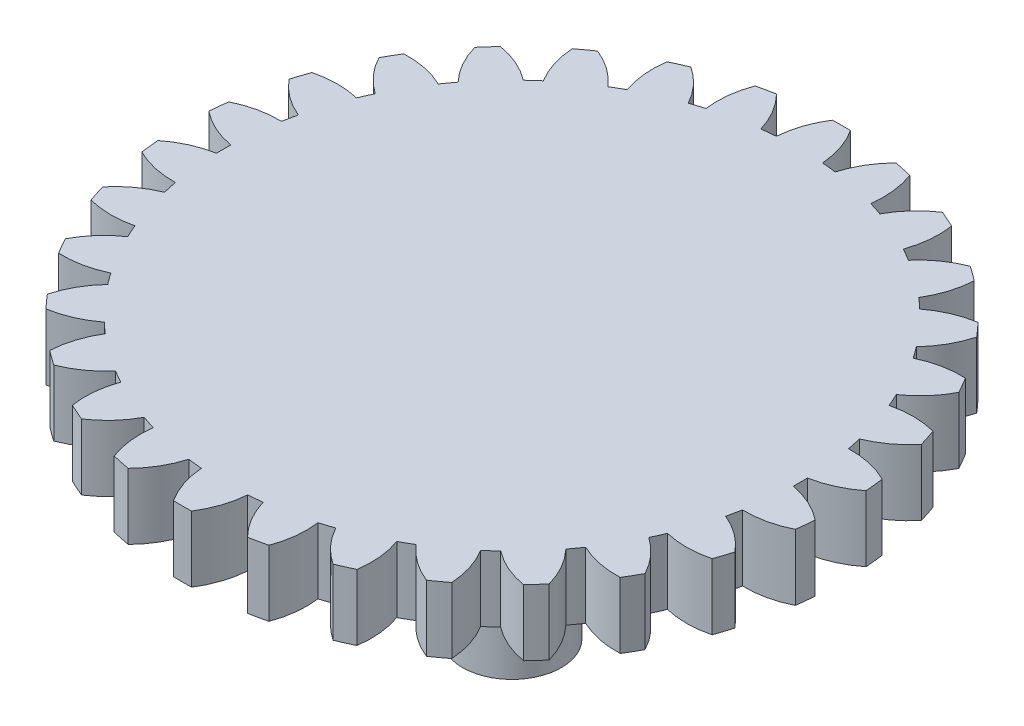
SolidWorks part; units mm, degrees
ref_plane "Front Plane" through (0, 0, 0) normal (0, 0, 1) x (1, 0, 0)
ref_plane "Top Plane" through (0, 0, 0) normal (0, 1, 0) x (1, 0, 0)
ref_plane "Right Plane" through (0, 0, 0) normal (1, 0, 0) x (0, 0, -1)
other "Configuration Table"
sketch "Sketch1" plane through (0, 0, 0) normal (0, 1, 0) x (1, 0, 0)
  circle A0 centre (0, 0) radius 30
  dimension "D1" = 60
extrude "Boss-Extrude1" add sketch "Sketch1" along normal blind 100
sketch "Sketch2" plane through (0, 100, 0) normal (0, 1, 0) x (1, 0, 0)
  circle A0 centre (0, 0) radius 50
  dimension "D1" = 100
extrude "Boss-Extrude2" add sketch "Sketch2" along normal blind 30
sketch "Sketch3" plane through (0, 130, 0) normal (0, 1, 0) x (1, 0, 0)
  line L0 (0, 0) -> (0, 200) construction
  line L1 (-18.2925, 174.0413) -> (0, 0) construction
  line L2 (0, 0) -> (18.2925, 174.0413) construction
  arc A0 (5.4995, 199.9244) -> (-5.4995, 199.9244) centre (0, 0) ccw
  arc A96 (-14, 174.4391) -> (-18.2925, 174.0413) centre (0, 0) ccw construction
  arc A97 (18.2925, 174.0413) -> (14, 174.4391) centre (0, 0) ccw construction
  arc A98 (-5.4995, 199.9244) -> (-14, 174.4391) centre (40.8445, 170.3062) ccw
  arc A99 (5.4995, 199.9244) -> (14, 174.4391) centre (-40.8445, 170.3062) cw
  arc A100 (36.1873, 196.699) -> (22.5739, 173.538) centre (75.3606, 158.0926) ccw
  arc A101 (46.9459, 194.4121) -> (36.1873, 196.699) centre (0, 0) ccw
  arc A102 (46.9459, 194.4121) -> (49.962, 167.7164) centre (-4.5433, 175.0767) cw
  arc A103 (76.2925, 184.8768) -> (58.1611, 165.0524) centre (106.5831, 138.9695) ccw
  arc A104 (86.3406, 180.4032) -> (76.2925, 184.8768) centre (0, 0) ccw
  arc A105 (86.3406, 180.4032) -> (83.7404, 153.6637) centre (31.9565, 172.1954) cw
  arc A106 (113.0634, 164.9747) -> (91.2065, 149.3532) centre (133.1474, 113.7728) ccw
  arc A107 (121.9618, 158.5097) -> (113.0634, 164.9747) centre (0, 0) ccw
  arc A108 (121.9618, 158.5097) -> (113.859, 132.8952) centre (67.0596, 161.7884) cw
  arc A109 (144.8929, 137.8624) -> (120.2657, 127.1266) centre (153.8925, 83.6037) ccw
  arc A110 (152.2526, 129.6886) -> (144.8929, 137.8624) centre (0, 0) ccw
  arc A111 (152.2526, 129.6886) -> (139.0013, 106.3185) centre (99.2319, 144.3105) cw
  arc A112 (170.3898, 104.7249) -> (144.0687, 99.3439) centre (167.9118, 49.7807) ccw
  arc A113 (175.8893, 95.1995) -> (170.3898, 104.7249) centre (0, 0) ccw
  arc A114 (175.8893, 95.1995) -> (158.0687, 75.0952) centre (127.0673, 120.5255) cw
  arc A115 (188.4399, 67.0103) -> (161.5752, 67.2194) centre (174.5925, 13.7821) ccw
  arc A116 (191.8388, 56.5497) -> (188.4399, 67.0103) centre (0, 0) ccw
  arc A117 (191.8388, 56.5497) -> (170.2277, 40.5899) centre (149.3492, 91.4729) cw
  arc A118 (198.2543, 26.3671) -> (172.0201, 32.1572) centre (173.6427, -22.8189) ccw
  arc A119 (199.404, 15.4284) -> (198.2543, 26.3671) centre (0, 0) ccw
  arc A120 (199.404, 15.4284) -> (174.9469, 4.3105) centre (165.1038, 58.4226) cw
  arc A121 (199.404, -15.4284) -> (174.9469, -4.3105) centre (165.1038, -58.4226) ccw
  arc A122 (198.2543, -26.3671) -> (199.404, -15.4284) centre (0, 0) ccw
  arc A123 (198.2543, -26.3671) -> (172.0201, -32.1572) centre (173.6427, 22.8189) cw
  arc A124 (191.8388, -56.5497) -> (170.2277, -40.5899) centre (149.3492, -91.4729) ccw
  arc A125 (188.4399, -67.0103) -> (191.8388, -56.5497) centre (0, 0) ccw
  arc A126 (188.4399, -67.0103) -> (161.5752, -67.2194) centre (174.5925, -13.7821) cw
  arc A127 (175.8893, -95.1995) -> (158.0687, -75.0952) centre (127.0673, -120.5255) ccw
  arc A128 (170.3898, -104.7249) -> (175.8893, -95.1995) centre (0, 0) ccw
  arc A129 (170.3898, -104.7249) -> (144.0687, -99.3439) centre (167.9118, -49.7807) cw
  arc A130 (152.2526, -129.6886) -> (139.0013, -106.3185) centre (99.2319, -144.3105) ccw
  arc A131 (144.8929, -137.8624) -> (152.2526, -129.6886) centre (0, 0) ccw
  arc A132 (144.8929, -137.8624) -> (120.2657, -127.1266) centre (153.8925, -83.6037) cw
  arc A133 (121.9618, -158.5097) -> (113.859, -132.8952) centre (67.0596, -161.7884) ccw
  arc A134 (113.0634, -164.9747) -> (121.9618, -158.5097) centre (0, 0) ccw
  arc A135 (113.0634, -164.9747) -> (91.2065, -149.3532) centre (133.1474, -113.7728) cw
  arc A136 (86.3406, -180.4032) -> (83.7404, -153.6637) centre (31.9565, -172.1954) ccw
  arc A137 (76.2925, -184.8768) -> (86.3406, -180.4032) centre (0, 0) ccw
  arc A138 (76.2925, -184.8768) -> (58.1611, -165.0524) centre (106.5831, -138.9695) cw
  arc A139 (46.9459, -194.4121) -> (49.962, -167.7164) centre (-4.5433, -175.0767) ccw
  arc A140 (36.1873, -196.699) -> (46.9459, -194.4121) centre (0, 0) ccw
  arc A141 (36.1873, -196.699) -> (22.5739, -173.538) centre (75.3606, -158.0926) cw
  arc A142 (5.4995, -199.9244) -> (14, -174.4391) centre (-40.8445, -170.3062) ccw
  arc A143 (-5.4995, -199.9244) -> (5.4995, -199.9244) centre (0, 0) ccw
  arc A144 (-5.4995, -199.9244) -> (-14, -174.4391) centre (40.8445, -170.3062) cw
  arc A145 (-36.1873, -196.699) -> (-22.5739, -173.538) centre (-75.3606, -158.0926) ccw
  arc A146 (-46.9459, -194.4121) -> (-36.1873, -196.699) centre (0, 0) ccw
  arc A147 (-46.9459, -194.4121) -> (-49.962, -167.7164) centre (4.5433, -175.0767) cw
  arc A148 (-76.2925, -184.8768) -> (-58.1611, -165.0524) centre (-106.5831, -138.9695) ccw
  arc A149 (-86.3406, -180.4032) -> (-76.2925, -184.8768) centre (0, 0) ccw
  arc A150 (-86.3406, -180.4032) -> (-83.7404, -153.6637) centre (-31.9565, -172.1954) cw
  arc A151 (-113.0634, -164.9747) -> (-91.2065, -149.3532) centre (-133.1474, -113.7728) ccw
  arc A152 (-121.9618, -158.5097) -> (-113.0634, -164.9747) centre (0, 0) ccw
  arc A153 (-121.9618, -158.5097) -> (-113.859, -132.8952) centre (-67.0596, -161.7884) cw
  arc A154 (-144.8929, -137.8624) -> (-120.2657, -127.1266) centre (-153.8925, -83.6037) ccw
  arc A155 (-152.2526, -129.6886) -> (-144.8929, -137.8624) centre (0, 0) ccw
  arc A156 (-152.2526, -129.6886) -> (-139.0013, -106.3185) centre (-99.2319, -144.3105) cw
  arc A157 (-170.3898, -104.7249) -> (-144.0687, -99.3439) centre (-167.9118, -49.7807) ccw
  arc A158 (-175.8893, -95.1995) -> (-170.3898, -104.7249) centre (0, 0) ccw
  arc A159 (-175.8893, -95.1995) -> (-158.0687, -75.0952) centre (-127.0673, -120.5255) cw
  arc A160 (-188.4399, -67.0103) -> (-161.5752, -67.2194) centre (-174.5925, -13.7821) ccw
  arc A161 (-191.8388, -56.5497) -> (-188.4399, -67.0103) centre (0, 0) ccw
  arc A162 (-191.8388, -56.5497) -> (-170.2277, -40.5899) centre (-149.3492, -91.4729) cw
  arc A163 (-198.2543, -26.3671) -> (-172.0201, -32.1572) centre (-173.6427, 22.8189) ccw
  arc A164 (-199.404, -15.4284) -> (-198.2543, -26.3671) centre (0, 0) ccw
  arc A165 (-199.404, -15.4284) -> (-174.9469, -4.3105) centre (-165.1038, -58.4226) cw
  arc A166 (-199.404, 15.4284) -> (-174.9469, 4.3105) centre (-165.1038, 58.4226) ccw
  arc A167 (-198.2543, 26.3671) -> (-199.404, 15.4284) centre (0, 0) ccw
  arc A168 (-198.2543, 26.3671) -> (-172.0201, 32.1572) centre (-173.6427, -22.8189) cw
  arc A169 (-191.8388, 56.5497) -> (-170.2277, 40.5899) centre (-149.3492, 91.4729) ccw
  arc A170 (-188.4399, 67.0103) -> (-191.8388, 56.5497) centre (0, 0) ccw
  arc A171 (-188.4399, 67.0103) -> (-161.5752, 67.2194) centre (-174.5925, 13.7821) cw
  arc A172 (-175.8893, 95.1995) -> (-158.0687, 75.0952) centre (-127.0673, 120.5255) ccw
  arc A173 (-170.3898, 104.7249) -> (-175.8893, 95.1995) centre (0, 0) ccw
  arc A174 (-170.3898, 104.7249) -> (-144.0687, 99.3439) centre (-167.9118, 49.7807) cw
  arc A175 (-152.2526, 129.6886) -> (-139.0013, 106.3185) centre (-99.2319, 144.3105) ccw
  arc A176 (-144.8929, 137.8624) -> (-152.2526, 129.6886) centre (0, 0) ccw
  arc A177 (-144.8929, 137.8624) -> (-120.2657, 127.1266) centre (-153.8925, 83.6037) cw
  arc A178 (-121.9618, 158.5097) -> (-113.859, 132.8952) centre (-67.0596, 161.7884) ccw
  arc A179 (-113.0634, 164.9747) -> (-121.9618, 158.5097) centre (0, 0) ccw
  arc A180 (-113.0634, 164.9747) -> (-91.2065, 149.3532) centre (-133.1474, 113.7728) cw
  arc A181 (-86.3406, 180.4032) -> (-83.7404, 153.6637) centre (-31.9565, 172.1954) ccw
  arc A182 (-76.2925, 184.8768) -> (-86.3406, 180.4032) centre (0, 0) ccw
  arc A183 (-76.2925, 184.8768) -> (-58.1611, 165.0524) centre (-106.5831, 138.9695) cw
  arc A184 (-46.9459, 194.4121) -> (-49.962, 167.7164) centre (4.5433, 175.0767) ccw
  arc A185 (-36.1873, 196.699) -> (-46.9459, 194.4121) centre (0, 0) ccw
  arc A186 (-36.1873, 196.699) -> (-22.5739, 173.538) centre (-75.3606, 158.0926) cw
  arc A187 (-49.962, 167.7164) -> (-58.1611, 165.0524) centre (0, 0) ccw
  arc A188 (-83.7404, 153.6637) -> (-91.2065, 149.3532) centre (0, 0) ccw
  arc A189 (-113.859, 132.8952) -> (-120.2657, 127.1266) centre (0, 0) ccw
  arc A190 (-139.0013, 106.3185) -> (-144.0687, 99.3439) centre (0, 0) ccw
  arc A191 (-158.0687, 75.0952) -> (-161.5752, 67.2194) centre (0, 0) ccw
  arc A192 (-170.2277, 40.5899) -> (-172.0201, 32.1572) centre (0, 0) ccw
  arc A193 (-174.9469, 4.3105) -> (-174.9469, -4.3105) centre (0, 0) ccw
  arc A194 (-172.0201, -32.1572) -> (-170.2277, -40.5899) centre (0, 0) ccw
  arc A195 (-161.5752, -67.2194) -> (-158.0687, -75.0952) centre (0, 0) ccw
  arc A196 (-144.0687, -99.3439) -> (-139.0013, -106.3185) centre (0, 0) ccw
  arc A197 (-120.2657, -127.1266) -> (-113.859, -132.8952) centre (0, 0) ccw
  arc A198 (-91.2065, -149.3532) -> (-83.7404, -153.6637) centre (0, 0) ccw
  arc A199 (-58.1611, -165.0524) -> (-49.962, -167.7164) centre (0, 0) ccw
  arc A200 (-22.5739, -173.538) -> (-14, -174.4391) centre (0, 0) ccw
  arc A201 (14, -174.4391) -> (22.5739, -173.538) centre (0, 0) ccw
  arc A202 (49.962, -167.7164) -> (58.1611, -165.0524) centre (0, 0) ccw
  arc A203 (83.7404, -153.6637) -> (91.2065, -149.3532) centre (0, 0) ccw
  arc A204 (113.859, -132.8952) -> (120.2657, -127.1266) centre (0, 0) ccw
  arc A205 (158.0687, -75.0952) -> (161.5752, -67.2194) centre (0, 0) ccw
  arc A206 (139.0013, -106.3185) -> (144.0687, -99.3439) centre (0, 0) ccw
  arc A207 (170.2277, -40.5899) -> (172.0201, -32.1572) centre (0, 0) ccw
  arc A208 (174.9469, -4.3105) -> (174.9469, 4.3105) centre (0, 0) ccw
  arc A209 (172.0201, 32.1572) -> (170.2277, 40.5899) centre (0, 0) ccw
  arc A210 (161.5752, 67.2194) -> (158.0687, 75.0952) centre (0, 0) ccw
  arc A211 (144.0687, 99.3439) -> (139.0013, 106.3185) centre (0, 0) ccw
  arc A212 (120.2657, 127.1266) -> (113.859, 132.8952) centre (0, 0) ccw
  arc A213 (91.2065, 149.3532) -> (83.7404, 153.6637) centre (0, 0) ccw
  arc A214 (58.1611, 165.0524) -> (49.962, 167.7164) centre (0, 0) ccw
  arc A215 (22.5739, 173.538) -> (14, 174.4391) centre (0, 0) ccw
  arc A216 (-14, 174.4391) -> (-22.5739, 173.538) centre (0, 0) ccw
  point P187 (0, 0)
  point P189 (0, 0)
  dimension "D2" = 175
  dimension "D9" = 14
  dimension "D10" = 55
  dimension "D12" = 55
  dimension "D6" = 200
  dimension "D5" = 14
  dimension "D3" = 5.5
  dimension "D4" = 5.5
  dimension "D7" = 6
  dimension "D8" = 6
extrude "Boss-Extrude3" add sketch "Sketch3" along normal blind 40 separate body
